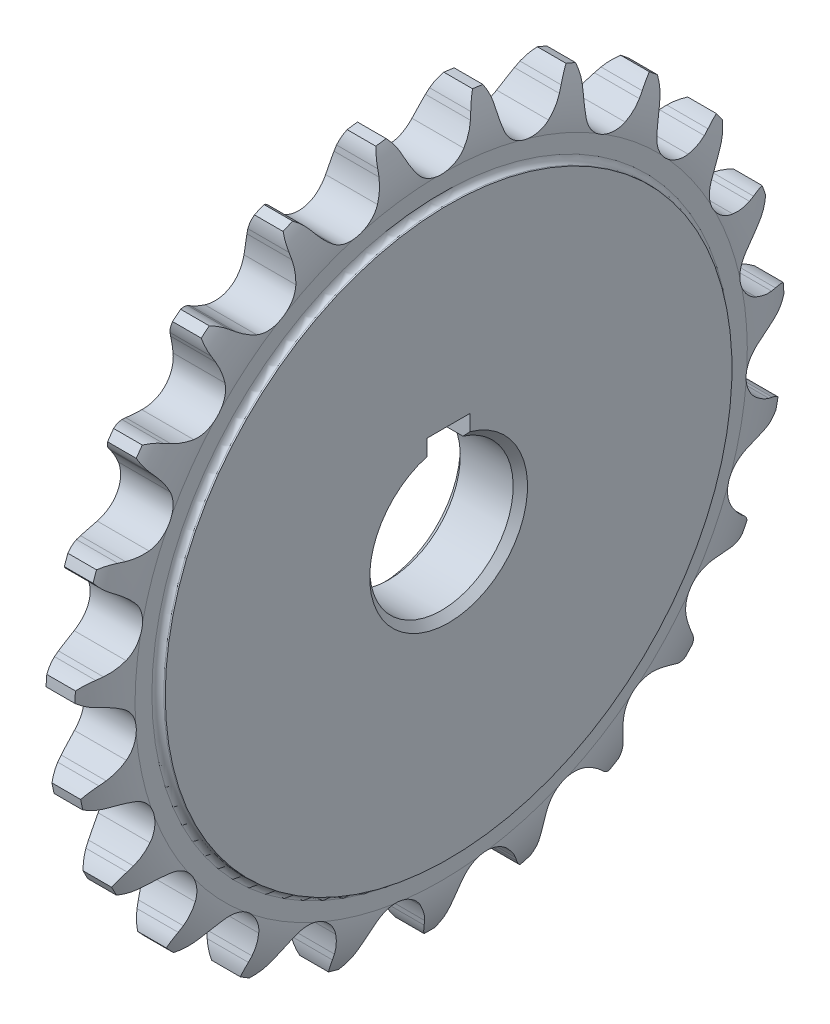
from build123d import *

# Parameters (mm, degrees)
CUT_EXTRUDE_1_DEPTH      = 4.685156443
PATTERN_CIRCULAR_1_COUNT = 23
SKETCH_4_W               = 6
SKETCH_4_H               = 3.260607938
CUT_EXTRUDE_2_DEPTH      = 71.578126957
CHAMFER_1_SIZE           = 1
CHAMFER_2_SIZE           = 1


with BuildPart() as part:
    # 草图1 → 旋转1 (revolve)
    with BuildSketch(Plane.XY, mode=Mode.PRIVATE) as revolve_1_sk:
        with BuildLine():
            Line((-4.685156443, 10), (-4.685156443, 39.5))
            Line((-4.685156443, 39.5), (-4.478175154, 39.5))
            ThreePointArc((-4.478175154, 39.5), (-3.892743663, 39.742493663), (-3.65025, 40.327925154))
            Line((-3.65025, 40.327925154), (-3.65025, 42.674032945))
            ThreePointArc((-3.65025, 42.674032945), (-3.305953661, 46.203405438), (-1.99925, 49.5))
            Line((-1.99925, 49.5), (1.99925, 49.5))
            ThreePointArc((1.99925, 49.5), (3.305953661, 46.203405438), (3.65025, 42.674032945))
            Line((3.65025, 42.674032945), (3.65025, 40.327925154))
            ThreePointArc((3.65025, 40.327925154), (3.892743663, 39.742493663), (4.478175154, 39.5))
            Line((4.478175154, 39.5), (4.685156443, 39.5))
            Line((4.685156443, 39.5), (4.685156443, 10))
            Line((4.685156443, 10), (-4.685156443, 10))
        make_face()
    revolve(revolve_1_sk.sketch.rotate(Axis((-6.35, 0, 0), (1, 0, 0)), 90), axis=Axis((-6.35, 0, 0), (1, 0, 0)))

    # 草图2 → 切除-拉伸1 (cut, symmetric)
    with BuildSketch(Plane(origin=(0, 0, 0), x_dir=(0, 0, -1), z_dir=(1, 0, 0))):
        with BuildLine():
            Line((4.588692581, 46.610285416), (4.899653292, 47.378261808))
            ThreePointArc((4.899653292, 47.378261808), (5.378614734, 48.306828579), (6.018529669, 49.132751812))
            ThreePointArc((6.018529669, 49.132751812), (0, 49.5), (-6.018529669, 49.132751812))
            ThreePointArc((-6.018529669, 49.132751812), (-5.378614734, 48.306828579), (-4.899653292, 47.378261808))
            Line((-4.899653292, 47.378261808), (-4.588692581, 46.610285416))
            ThreePointArc((-4.588692581, 46.610285416), (-3.973376288, 45.345046883), (-3.192395607, 44.174785433))
            ThreePointArc((-3.192395607, 44.174785433), (0, 42.604232945), (3.192395607, 44.174785433))
            ThreePointArc((3.192395607, 44.174785433), (3.973376288, 45.345046883), (4.588692581, 46.610285416))
        make_face()
    cut_extrude_1 = extrude(amount=CUT_EXTRUDE_1_DEPTH, both=True, mode=Mode.SUBTRACT)

    # 阵列(圆周)1: 切除-拉伸1 ×23 about axis
    pattern_circular_1_axis = Axis((0, 0, 0), (1, 0, 0))
    for i in range(1, PATTERN_CIRCULAR_1_COUNT):
        add(cut_extrude_1.rotate(pattern_circular_1_axis, i * 360 / PATTERN_CIRCULAR_1_COUNT), mode=Mode.SUBTRACT)

    # 草图4 → 切除-拉伸2 (cut, through all)
    with BuildSketch(Plane.ZY.offset(4.685156443)):
        with Locations((0, 11.169695983)):
            Rectangle(SKETCH_4_W, SKETCH_4_H)
    extrude(amount=-CUT_EXTRUDE_2_DEPTH, mode=Mode.SUBTRACT)

    # 倒角1
    chamfer_1_edges = [part.edges().sort_by_distance(p)[0] for p in [
        (-4.685156443, -10, 0),
    ]]
    chamfer(chamfer_1_edges, length=CHAMFER_1_SIZE)

    # 倒角2
    chamfer_2_edges = [part.edges().sort_by_distance(p)[0] for p in [
        (4.685156443, -10, 0),
    ]]
    chamfer(chamfer_2_edges, length=CHAMFER_2_SIZE)


solid = part.part
